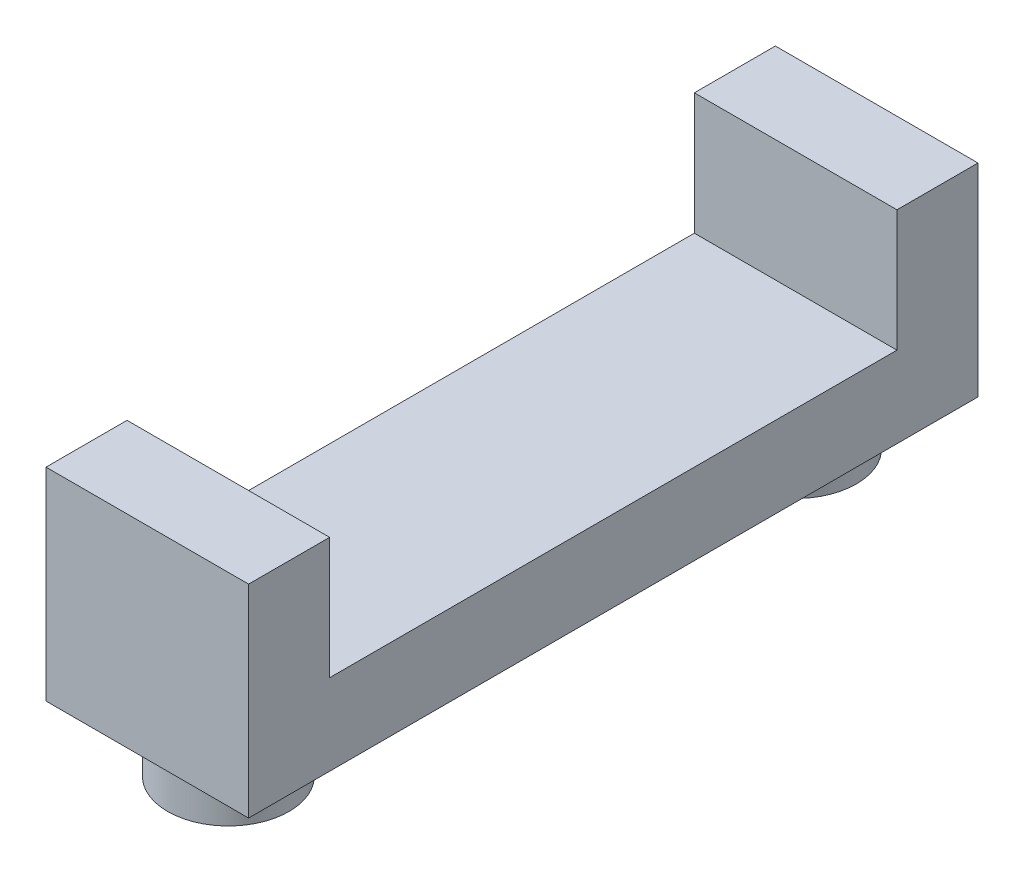
SolidWorks part; units mm, degrees
ref_plane "Front Plane" through (0, 0, 0) normal (0, 0, 1) x (1, 0, 0)
ref_plane "Top Plane" through (0, 0, 0) normal (0, 1, 0) x (1, 0, 0)
ref_plane "Right Plane" through (0, 0, 0) normal (1, 0, 0) x (0, 0, -1)
sketch "Sketch1" plane through (0, 0, 0) normal (0, 0, 1) x (1, 0, 0)
  line L1 (-250, -250) -> (250, -250)
  line L2 (-250, -250) -> (-250, 250)
  line L3 (-250, 250) -> (250, 250)
  line L4 (250, -250) -> (250, 250)
  line L5 (-250, -250) -> (250, 250) construction
  line L6 (-250, 250) -> (250, -250) construction
  point P0 (0, 0)
  dimension "D1" = 500
  dimension "D2" = 500
extrude "Boss-Extrude1" add sketch "Sketch1" along normal mid plane 1800
sketch "Sketch2" plane through (0, -250, 0) normal (0, -1, 0) x (1, 0, 0)
  line L0 (0, 0) -> (-386.5993, 0) construction
  line L1 (0, -700) -> (0, 0) construction
  circle A0 centre (0, -700) radius 150
  circle A1 centre (0, 700) radius 150
  dimension "D1" = 300
  dimension "D2" = 1400
extrude "Boss-Extrude2" add sketch "Sketch2" along normal blind 136
sketch "Sketch3" plane through (250, 0, 0) normal (1, 0, 0) x (0, 0, -1)
  line L0 (-900, 250) -> (900, 250) construction
  line L1 (-700, 250) -> (700, 250)
  line L2 (-700, 250) -> (-700, -50)
  line L3 (-700, -50) -> (700, -50)
  line L4 (700, 250) -> (700, -50)
  line L5 (0, 0) -> (0, 362.8061) construction
  dimension "D1" = 1400
  dimension "D2" = 300
extrude "Cut-Extrude1" cut sketch "Sketch3" against normal through all
